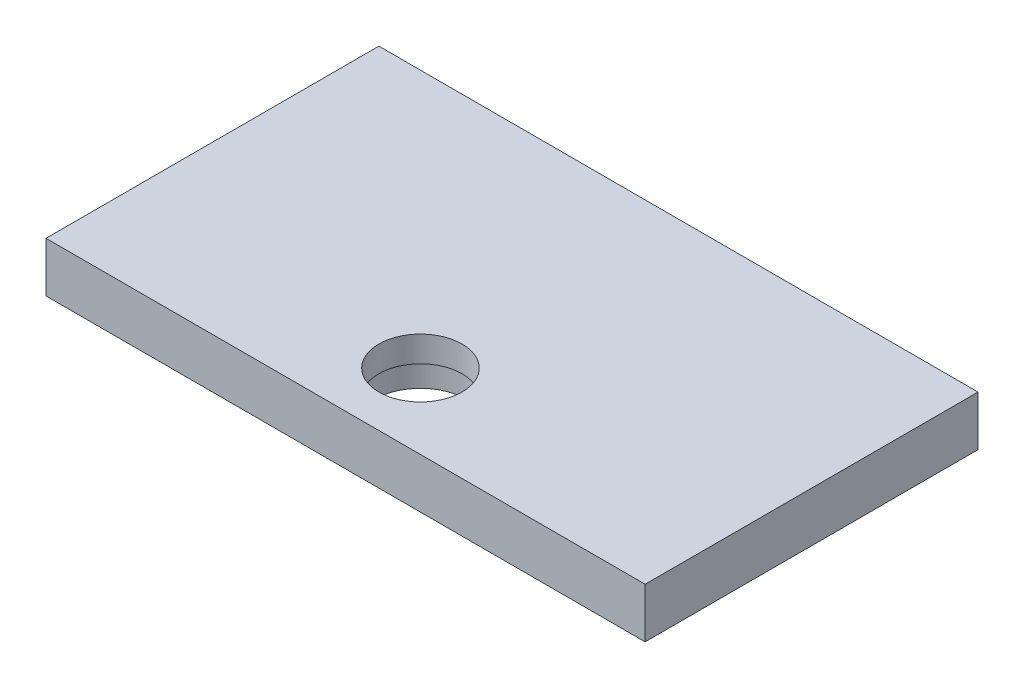
SolidWorks part; units mm, degrees
ref_plane "前视基准面" through (0, 0, 0) normal (0, 0, 1) x (1, 0, 0)
ref_plane "上视基准面" through (0, 0, 0) normal (0, 1, 0) x (1, 0, 0)
ref_plane "右视基准面" through (0, 0, 0) normal (1, 0, 0) x (0, 0, -1)
sketch "草图1" plane through (0, 0, 0) normal (0, 1, 0) x (1, 0, 0)
  line L1 (-180, -100) -> (180, -100)
  line L2 (-180, -100) -> (-180, 100)
  line L3 (-180, 100) -> (180, 100)
  line L4 (180, -100) -> (180, 100)
  line L5 (-180, -100) -> (180, 100) construction
  line L6 (-180, 100) -> (180, -100) construction
  point P0 (0, 0)
  dimension "D1" = 200
  dimension "D2" = 360
extrude "凸台-拉伸1" add sketch "草图1" along normal blind 30
sketch "草图2" plane through (0, 0, 0) normal (0, -1, 0) x (1, 0, 0)
  line L0 (180, 100) -> (180, -100) construction
  line L1 (-180, 100) -> (180, 100) construction
  circle A0 centre (0, 55) radius 25
  dimension "D1" = 50
  dimension "D2" = 180
  dimension "D3" = 45
extrude "切除-拉伸1" cut sketch "草图2" against normal through all
sketch "草图3" plane through (0, 0, 0) normal (0, -1, 0) x (1, 0, 0)
  line L0 (180, 100) -> (180, -100) construction
  line L1 (-180, 100) -> (180, 100) construction
  circle A0 centre (0, 55) radius 27.5
  dimension "D1" = 55
  dimension "D2" = 180
  dimension "D3" = 45
extrude "切除-拉伸2" cut sketch "草图3" against normal blind 14.53
